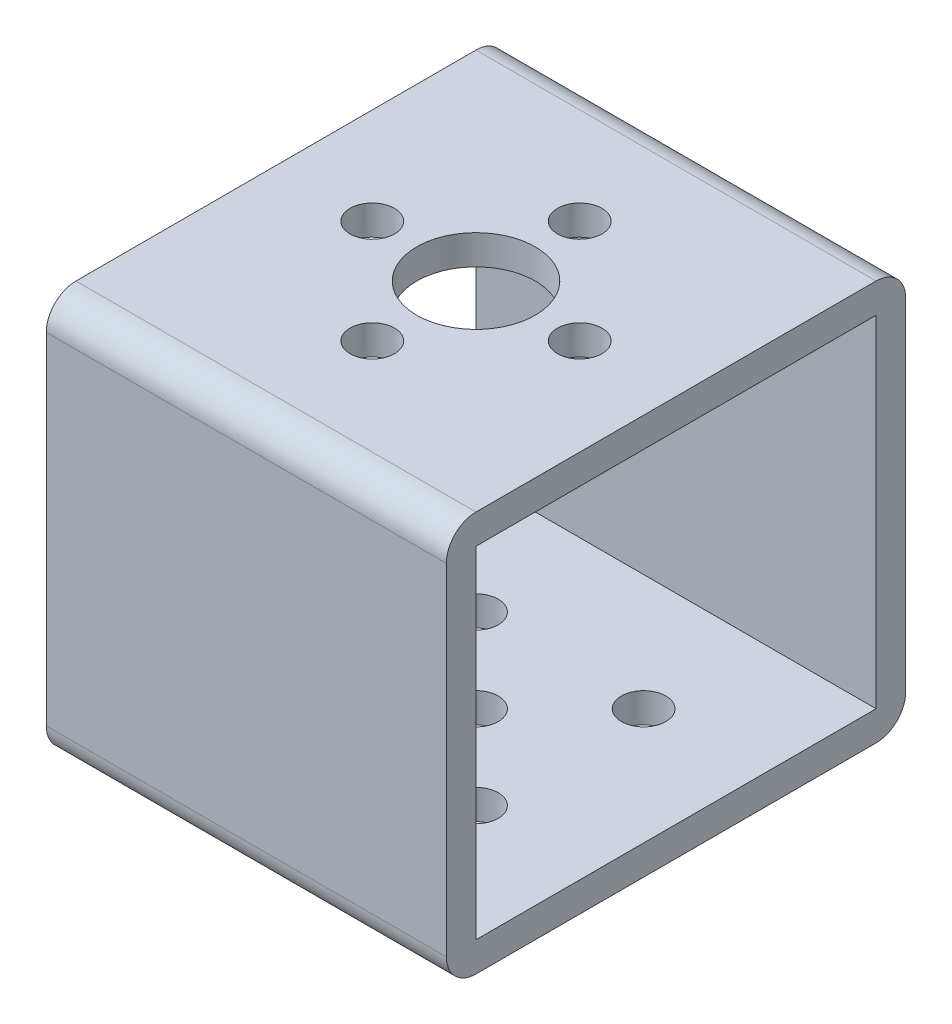
from build123d import *

# Parameters (mm, degrees)
SKETCH1_W           = 27
SKETCH1_H           = 27
BOSS_EXTRUDE1_DEPTH = 29
SKETCH2_W           = 27
SKETCH2_H           = 23
CUT_EXTRUDE1_DEPTH  = 27
CUT_EXTRUDE2_REACH  = 43.86
SKETCH4_R           = 4
SKETCH4_R_2         = 1.5
CUT_EXTRUDE3_REACH  = 43.86
SKETCH5_R           = 1.5
FILLET1_R           = 2
SKETCH6_W           = 27
SKETCH6_H           = 2
BOSS_EXTRUDE2_DEPTH = 27
FILLET2_R           = 2


with BuildPart() as part:
    # Sketch1 → Boss-Extrude1 (new body)
    with BuildSketch(Plane.XY):
        Rectangle(SKETCH1_W, SKETCH1_H)
    extrude(amount=BOSS_EXTRUDE1_DEPTH)

    # Sketch2 → Cut-Extrude1 (cut)
    with BuildSketch(Plane(origin=(13.5, 0, 0), x_dir=(0, 0, -1), z_dir=(1, 0, 0))):
        with Locations((-15.5, 0)):
            Rectangle(SKETCH2_W, SKETCH2_H)
    extrude(amount=-CUT_EXTRUDE1_DEPTH, mode=Mode.SUBTRACT)

    # Sketch4 → Cut-Extrude2 (cut, up to next)
    with BuildSketch(Plane(origin=(0, 13.5, 0), x_dir=(1, 0, 0), z_dir=(0, 1, 0)), mode=Mode.PRIVATE) as cut_extrude2_sk1:
        with Locations(Location((0, -15.5, 0), (0, 0, 270))):
            Circle(SKETCH4_R)
    cut_extrude2_tool1 = extrude(cut_extrude2_sk1.sketch, amount=-CUT_EXTRUDE2_REACH, mode=Mode.PRIVATE) & part.part
    # Sketch4 → Cut-Extrude2 (cut, up to next)
    with BuildSketch(Plane(origin=(0, 13.5, 0), x_dir=(1, 0, 0), z_dir=(0, 1, 0)), mode=Mode.PRIVATE) as cut_extrude2_sk2:
        with Locations(Location((0, -8.5, 0), (0, 0, 270))):
            Circle(SKETCH4_R_2)
    cut_extrude2_tool2 = extrude(cut_extrude2_sk2.sketch, amount=-CUT_EXTRUDE2_REACH, mode=Mode.PRIVATE) & part.part
    # Sketch4 → Cut-Extrude2 (cut, up to next)
    with BuildSketch(Plane(origin=(0, 13.5, 0), x_dir=(1, 0, 0), z_dir=(0, 1, 0)), mode=Mode.PRIVATE) as cut_extrude2_sk3:
        with Locations(Location((7, -15.5, 0), (0, 0, 270))):
            Circle(SKETCH4_R_2)
    cut_extrude2_tool3 = extrude(cut_extrude2_sk3.sketch, amount=-CUT_EXTRUDE2_REACH, mode=Mode.PRIVATE) & part.part
    # Sketch4 → Cut-Extrude2 (cut, up to next)
    with BuildSketch(Plane(origin=(0, 13.5, 0), x_dir=(1, 0, 0), z_dir=(0, 1, 0)), mode=Mode.PRIVATE) as cut_extrude2_sk4:
        with Locations(Location((0, -22.5, 0), (0, 0, 270))):
            Circle(SKETCH4_R_2)
    cut_extrude2_tool4 = extrude(cut_extrude2_sk4.sketch, amount=-CUT_EXTRUDE2_REACH, mode=Mode.PRIVATE) & part.part
    # Sketch4 → Cut-Extrude2 (cut, up to next)
    with BuildSketch(Plane(origin=(0, 13.5, 0), x_dir=(1, 0, 0), z_dir=(0, 1, 0)), mode=Mode.PRIVATE) as cut_extrude2_sk5:
        with Locations(Location((-7, -15.5, 0), (0, 0, 270))):
            Circle(SKETCH4_R_2)
    cut_extrude2_tool5 = extrude(cut_extrude2_sk5.sketch, amount=-CUT_EXTRUDE2_REACH, mode=Mode.PRIVATE) & part.part
    add(cut_extrude2_tool1.solids().sort_by_distance((0, 13.5, 15.5))[0], mode=Mode.SUBTRACT)
    add(cut_extrude2_tool2.solids().sort_by_distance((0, 13.5, 8.5))[0], mode=Mode.SUBTRACT)
    add(cut_extrude2_tool3.solids().sort_by_distance((7, 13.5, 15.5))[0], mode=Mode.SUBTRACT)
    add(cut_extrude2_tool4.solids().sort_by_distance((0, 13.5, 22.5))[0], mode=Mode.SUBTRACT)
    add(cut_extrude2_tool5.solids().sort_by_distance((-7, 13.5, 15.5))[0], mode=Mode.SUBTRACT)

    # Sketch5 → Cut-Extrude3 (cut, up to next)
    with BuildSketch(Plane.XZ.offset(13.5), mode=Mode.PRIVATE) as cut_extrude3_sk1:
        with Locations(Location((0, 15.5, 0), (0, 0, 270))):
            Circle(SKETCH5_R)
    cut_extrude3_tool1 = extrude(cut_extrude3_sk1.sketch, amount=-CUT_EXTRUDE3_REACH, mode=Mode.PRIVATE) & part.part
    # Sketch5 → Cut-Extrude3 (cut, up to next)
    with BuildSketch(Plane.XZ.offset(13.5), mode=Mode.PRIVATE) as cut_extrude3_sk2:
        with Locations(Location((-5.656854249, 21.156854249, 0), (0, 0, 270))):
            Circle(SKETCH5_R)
    cut_extrude3_tool2 = extrude(cut_extrude3_sk2.sketch, amount=-CUT_EXTRUDE3_REACH, mode=Mode.PRIVATE) & part.part
    # Sketch5 → Cut-Extrude3 (cut, up to next)
    with BuildSketch(Plane.XZ.offset(13.5), mode=Mode.PRIVATE) as cut_extrude3_sk3:
        with Locations(Location((5.656854249, 21.156854249, 0), (0, 0, 270))):
            Circle(SKETCH5_R)
    cut_extrude3_tool3 = extrude(cut_extrude3_sk3.sketch, amount=-CUT_EXTRUDE3_REACH, mode=Mode.PRIVATE) & part.part
    # Sketch5 → Cut-Extrude3 (cut, up to next)
    with BuildSketch(Plane.XZ.offset(13.5), mode=Mode.PRIVATE) as cut_extrude3_sk4:
        with Locations(Location((5.656854249, 9.843145751, 0), (0, 0, 270))):
            Circle(SKETCH5_R)
    cut_extrude3_tool4 = extrude(cut_extrude3_sk4.sketch, amount=-CUT_EXTRUDE3_REACH, mode=Mode.PRIVATE) & part.part
    # Sketch5 → Cut-Extrude3 (cut, up to next)
    with BuildSketch(Plane.XZ.offset(13.5), mode=Mode.PRIVATE) as cut_extrude3_sk5:
        with Locations(Location((-5.656854249, 9.843145751, 0), (0, 0, 270))):
            Circle(SKETCH5_R)
    cut_extrude3_tool5 = extrude(cut_extrude3_sk5.sketch, amount=-CUT_EXTRUDE3_REACH, mode=Mode.PRIVATE) & part.part
    add(cut_extrude3_tool1.solids().sort_by_distance((0, -13.5, 15.5))[0], mode=Mode.SUBTRACT)
    add(cut_extrude3_tool2.solids().sort_by_distance((-5.656854, -13.5, 21.156854))[0], mode=Mode.SUBTRACT)
    add(cut_extrude3_tool3.solids().sort_by_distance((5.656854, -13.5, 21.156854))[0], mode=Mode.SUBTRACT)
    add(cut_extrude3_tool4.solids().sort_by_distance((5.656854, -13.5, 9.843146))[0], mode=Mode.SUBTRACT)
    add(cut_extrude3_tool5.solids().sort_by_distance((-5.656854, -13.5, 9.843146))[0], mode=Mode.SUBTRACT)

    # Fillet1
    fillet1_edges = [part.edges().sort_by_distance(p)[0] for p in [
        (0, -13.5, 0),
        (0, 13.5, 0),
    ]]
    fillet(fillet1_edges, radius=FILLET1_R)

    # Sketch6 → Boss-Extrude2 (add)
    with BuildSketch(Plane.XZ.offset(13.5)):
        with Locations((0, 30)):
            Rectangle(SKETCH6_W, SKETCH6_H)
    extrude(amount=-BOSS_EXTRUDE2_DEPTH)

    # Fillet2
    fillet2_edges = [part.edges().sort_by_distance(p)[0] for p in [
        (0, -13.5, 31),
        (0, 13.5, 31),
    ]]
    fillet(fillet2_edges, radius=FILLET2_R)


solid = part.part
